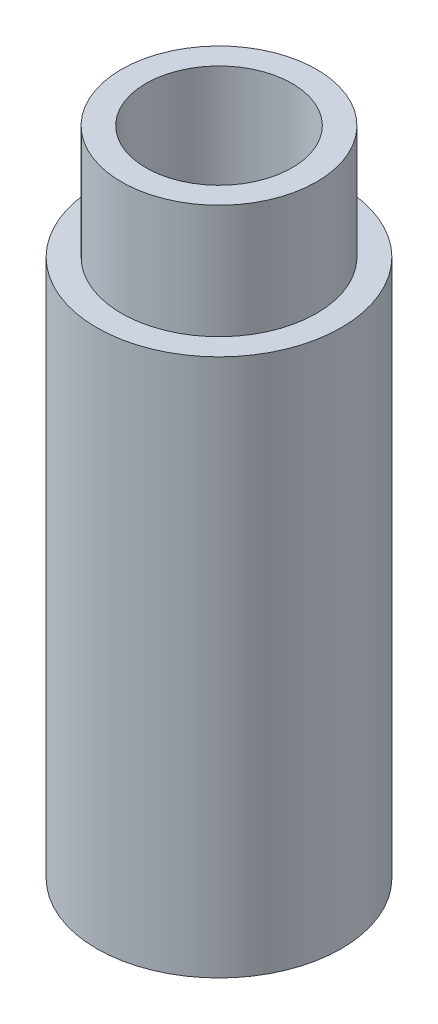
SolidWorks part; units mm, degrees
ref_plane "Plan de face" through (0, 0, 0) normal (0, 0, 1) x (1, 0, 0)
ref_plane "Plan de dessus" through (0, 0, 0) normal (0, 1, 0) x (1, 0, 0)
ref_plane "Plan de droite" through (0, 0, 0) normal (1, 0, 0) x (0, 0, -1)
sketch "Sketch2" plane through (0, 0, 0) normal (0, 0, 1) x (1, 0, 0)
  line L0 (71.0674, 101.1777) -> (71.0674, 20.6124) construction
  line L1 (51.0674, -25.4888) -> (51.0674, 80.0612)
  line L2 (51.0674, 80.0612) -> (56.1174, 80.0612)
  line L3 (56.1174, 80.0612) -> (56.1174, 107.7912)
  line L4 (46.0674, -25.4888) -> (46.0674, 84.5112)
  line L5 (38.9957, 75.0612) -> (61.3358, 75.0612) construction
  line L6 (51.1174, 97.7912) -> (51.1174, 107.7912)
  line L7 (51.0674, -25.4888) -> (46.0674, -25.4888)
  line L8 (51.1174, 107.7912) -> (56.1174, 107.7912)
  line L9 (46.0674, -25.4888) -> (46.0674, 95.7912) construction
  line L10 (46.0674, 95.7912) -> (51.1174, 95.7912) construction
  line L11 (51.1174, 84.5112) -> (46.0674, 84.5112)
  line L12 (51.0674, 90.7912) -> (56.1174, 90.7912) construction
  line L13 (56.1174, 90.7912) -> (56.1174, 107.7912) construction
  line L15 (51.0674, -25.4888) -> (51.0674, 90.7912) construction
  line L16 (51.1174, 95.7912) -> (51.1174, 107.7912) construction
  line L17 (51.1174, 84.5112) -> (51.1174, 97.7912)
  point P14 (52.5621, 97.0683)
  dimension "D1" = 20
  dimension "D2" = 14.95
  dimension "D3" = 5
  dimension "D4" = 23.28
  dimension "D6" = 27.73
  dimension "D7" = 110
  dimension "D5" = 5
revolve "Revolve1" add sketch "Sketch2" angle 360 about L0
